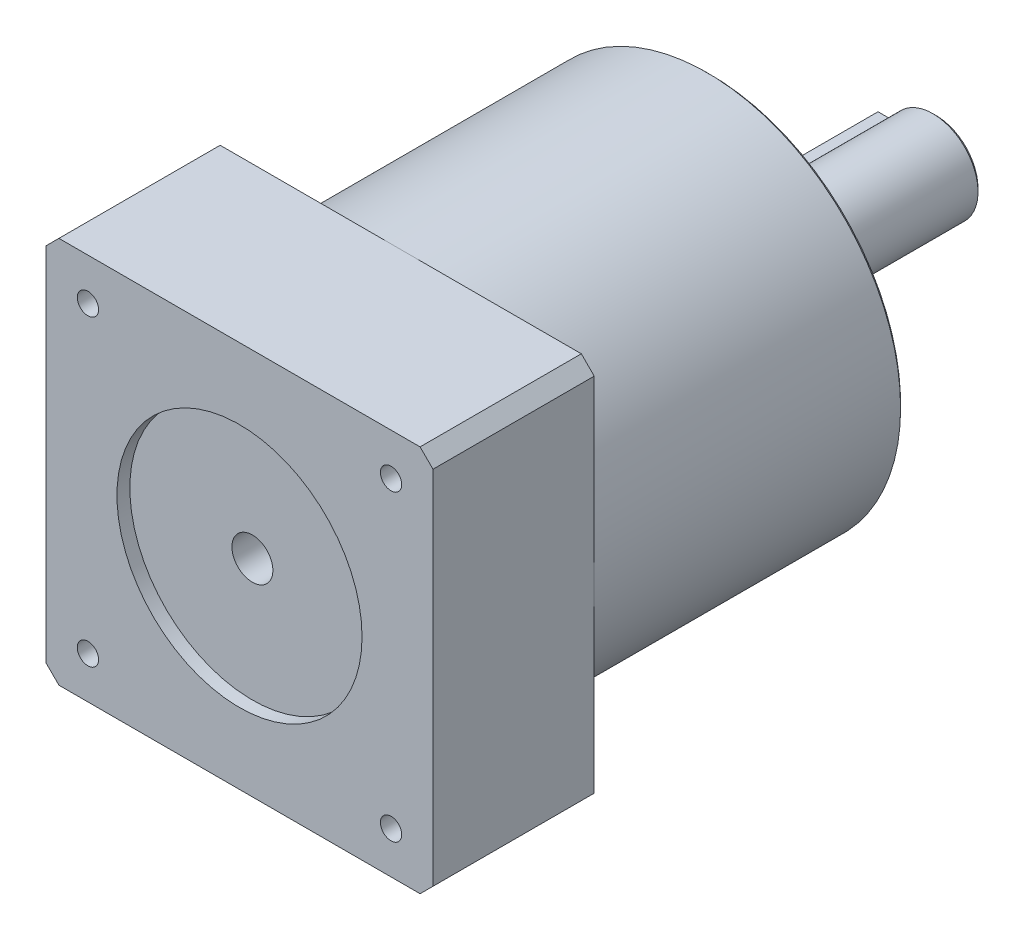
from build123d import *

# Parameters (mm, degrees)
SKETCH_1_W               = 60
SKETCH_1_H               = 60
EXTRUDE_1_DEPTH          = 25
SKETCH_2_R               = 30
EXTRUDE_2_DEPTH          = 48
SKETCH_3_R               = 20
EXTRUDE_3_DEPTH          = 3
SKETCH_4_R               = 8.5
EXTRUDE_4_DEPTH          = 2
SKETCH_5_R               = 7
EXTRUDE_5_DEPTH          = 30
SKETCH_7_R               = 3.175
CUT_EXTRUDE_1_DEPTH      = 21
SKETCH_8_R               = 19
CUT_EXTRUDE_2_DEPTH      = 2
PATTERN_CIRCULAR_1_COUNT = 4
CHAMFER_1_SIZE           = 2
SKETCH_17_W              = 4
SKETCH_17_H              = 5
EXTRUDE_6_DEPTH          = 27.5
CHAMFER_2_SIZE           = 0.5


with BuildPart() as part:
    # 草图1 → 凸台-拉伸1 (new body)
    with BuildSketch(Plane.XY):
        Rectangle(SKETCH_1_W, SKETCH_1_H)
    extrude(amount=EXTRUDE_1_DEPTH)

    # 草图2 → 凸台-拉伸2 (add)
    with BuildSketch(Plane(origin=(0, 0, 0), x_dir=(-1, 0, 0), z_dir=(0, 0, -1))):
        Circle(SKETCH_2_R)
    extrude(amount=EXTRUDE_2_DEPTH)

    # 草图3 → 凸台-拉伸3 (add)
    with BuildSketch(Plane(origin=(0, 0, -48), x_dir=(-1, 0, 0), z_dir=(0, 0, -1))):
        Circle(SKETCH_3_R)
    extrude(amount=EXTRUDE_3_DEPTH)

    # 草图4 → 凸台-拉伸4 (add)
    with BuildSketch(Plane(origin=(0, 0, -51), x_dir=(-1, 0, 0), z_dir=(0, 0, -1))):
        Circle(SKETCH_4_R)
    extrude(amount=EXTRUDE_4_DEPTH)

    # 草图5 → 凸台-拉伸5 (add)
    with BuildSketch(Plane(origin=(0, 0, -53), x_dir=(-1, 0, 0), z_dir=(0, 0, -1))):
        Circle(SKETCH_5_R)
    extrude(amount=EXTRUDE_5_DEPTH)

    # 草图7 → 切除-拉伸1 (cut)
    with BuildSketch(Plane.XY.offset(25)):
        Circle(SKETCH_7_R)
    extrude(amount=-CUT_EXTRUDE_1_DEPTH, mode=Mode.SUBTRACT)

    # 草图8 → 切除-拉伸2 (cut)
    with BuildSketch(Plane.XY.offset(25)):
        Circle(SKETCH_8_R)
    extrude(amount=-CUT_EXTRUDE_2_DEPTH, mode=Mode.SUBTRACT)

    # 草图10 → M4 螺纹孔1 (revolve, cut)
    with BuildSketch(Plane(origin=(23.5, 23.5, 25), x_dir=(0, -1, 0), z_dir=(1, 0, 0))):
        Polygon((0, 0), (0, 12.491420021), (1.65, 11.5), (1.65, 0), align=None)
    hole_wizard_m4_1 = revolve(axis=Axis((23.5, 23.5, 31.35), (0, 0, -1)), mode=Mode.SUBTRACT)

    # 草图15 → M5 螺纹孔1 (revolve, cut)
    with BuildSketch(Plane(origin=(-18.384776311, 18.384776311, -48), x_dir=(0, 1, 0), z_dir=(1, 0, 0))):
        Polygon((0, 0), (0, 13.2618073), (2.1, 12), (2.1, 0), align=None)
    hole_wizard_m5_1 = revolve(axis=Axis((-18.384776311, 18.384776311, -54.35), (0, 0, 1)), mode=Mode.SUBTRACT)

    # 阵列(圆周)1: M4 螺纹孔1, M5 螺纹孔1 ×4 about axis
    pattern_circular_1_axis = Axis((0, 0, 0), (0, 0, 1))
    add([hole_wizard_m4_1.rotate(pattern_circular_1_axis, i * 360 / PATTERN_CIRCULAR_1_COUNT) for i in range(1, PATTERN_CIRCULAR_1_COUNT)], mode=Mode.SUBTRACT)
    add([hole_wizard_m5_1.rotate(pattern_circular_1_axis, i * 360 / PATTERN_CIRCULAR_1_COUNT) for i in range(1, PATTERN_CIRCULAR_1_COUNT)], mode=Mode.SUBTRACT)

    # 倒角1
    chamfer_1_edges = [part.edges().sort_by_distance(p)[0] for p in [
        (30, -30, 12.5),
        (-30, -30, 12.5),
        (-30, 30, 12.5),
        (30, 30, 12.5),
    ]]
    chamfer(chamfer_1_edges, length=CHAMFER_1_SIZE)

    # 草图17 → 凸台-拉伸6 (add)
    with BuildSketch(Plane(origin=(0, 0, -83), x_dir=(-1, 0, 0), z_dir=(0, 0, -1))):
        with Locations((7, 0)):
            Rectangle(SKETCH_17_W, SKETCH_17_H)
    extrude(amount=-EXTRUDE_6_DEPTH)

    # 倒角2
    chamfer_2_edges = [part.edges().sort_by_distance(p)[0] for p in [
        (30, 0, -48),
        (7, 0, -83),
    ]]
    chamfer(chamfer_2_edges, length=CHAMFER_2_SIZE)


solid = part.part
